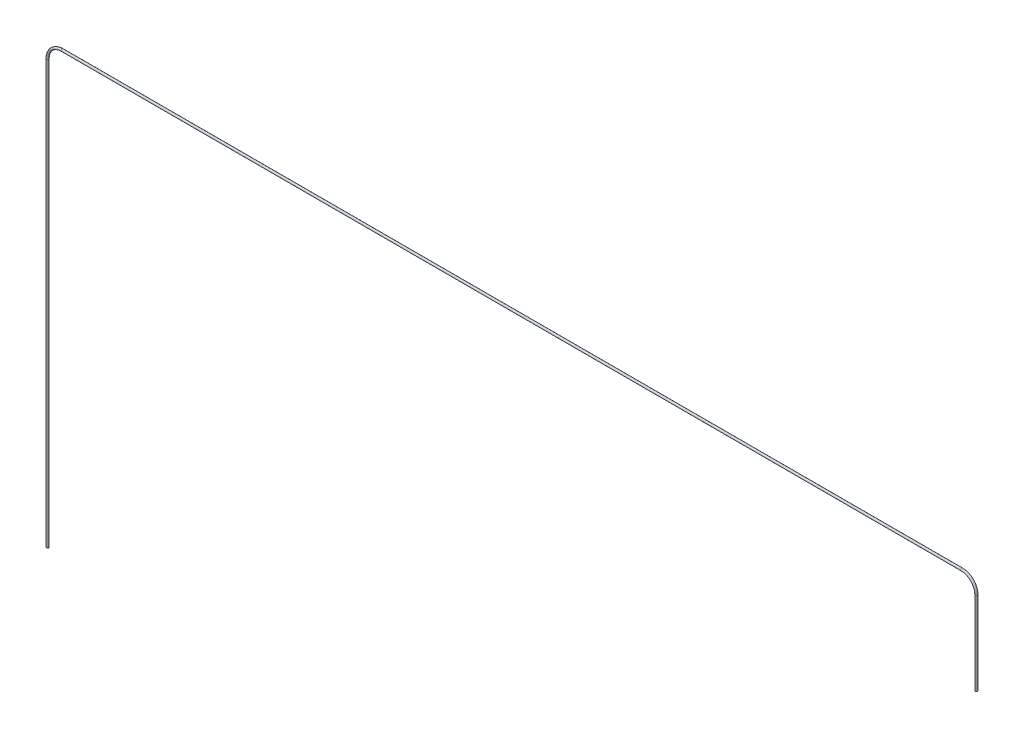
SolidWorks part; units mm, degrees
ref_plane "Front Plane" through (0, 0, 0) normal (0, 0, 1) x (1, 0, 0)
ref_plane "Top Plane" through (0, 0, 0) normal (0, 1, 0) x (1, 0, 0)
ref_plane "Right Plane" through (0, 0, 0) normal (1, 0, 0) x (0, 0, -1)
sketch "Sketch1" plane through (0, 0, 0) normal (0, 0, 1) x (1, 0, 0)
  line L0 (0, 0) -> (0, 1213)
  line L1 (42, 1255) -> (2620, 1255)
  line L2 (2662, 1213) -> (2662, 975)
  arc A0 (2620, 1255) -> (2662, 1213) centre (2620, 1213) cw
  arc A1 (0, 1213) -> (42, 1255) centre (42, 1213) cw
  point P7 (2662, 1255)
  point P10 (0, 1255)
  dimension "D3" = 42
  dimension "D1" = 2662
  dimension "D2" = 1255
  dimension "D4" = 280
sketch "Sketch2" plane through (0, 0, 0) normal (0, 1, 0) x (1, 0, 0)
  circle A0 centre (0, 0) radius 3.25
  dimension "D1" = 6.5
sweep "Sweep1" add profiles "Sketch2" path "Sketch1"
